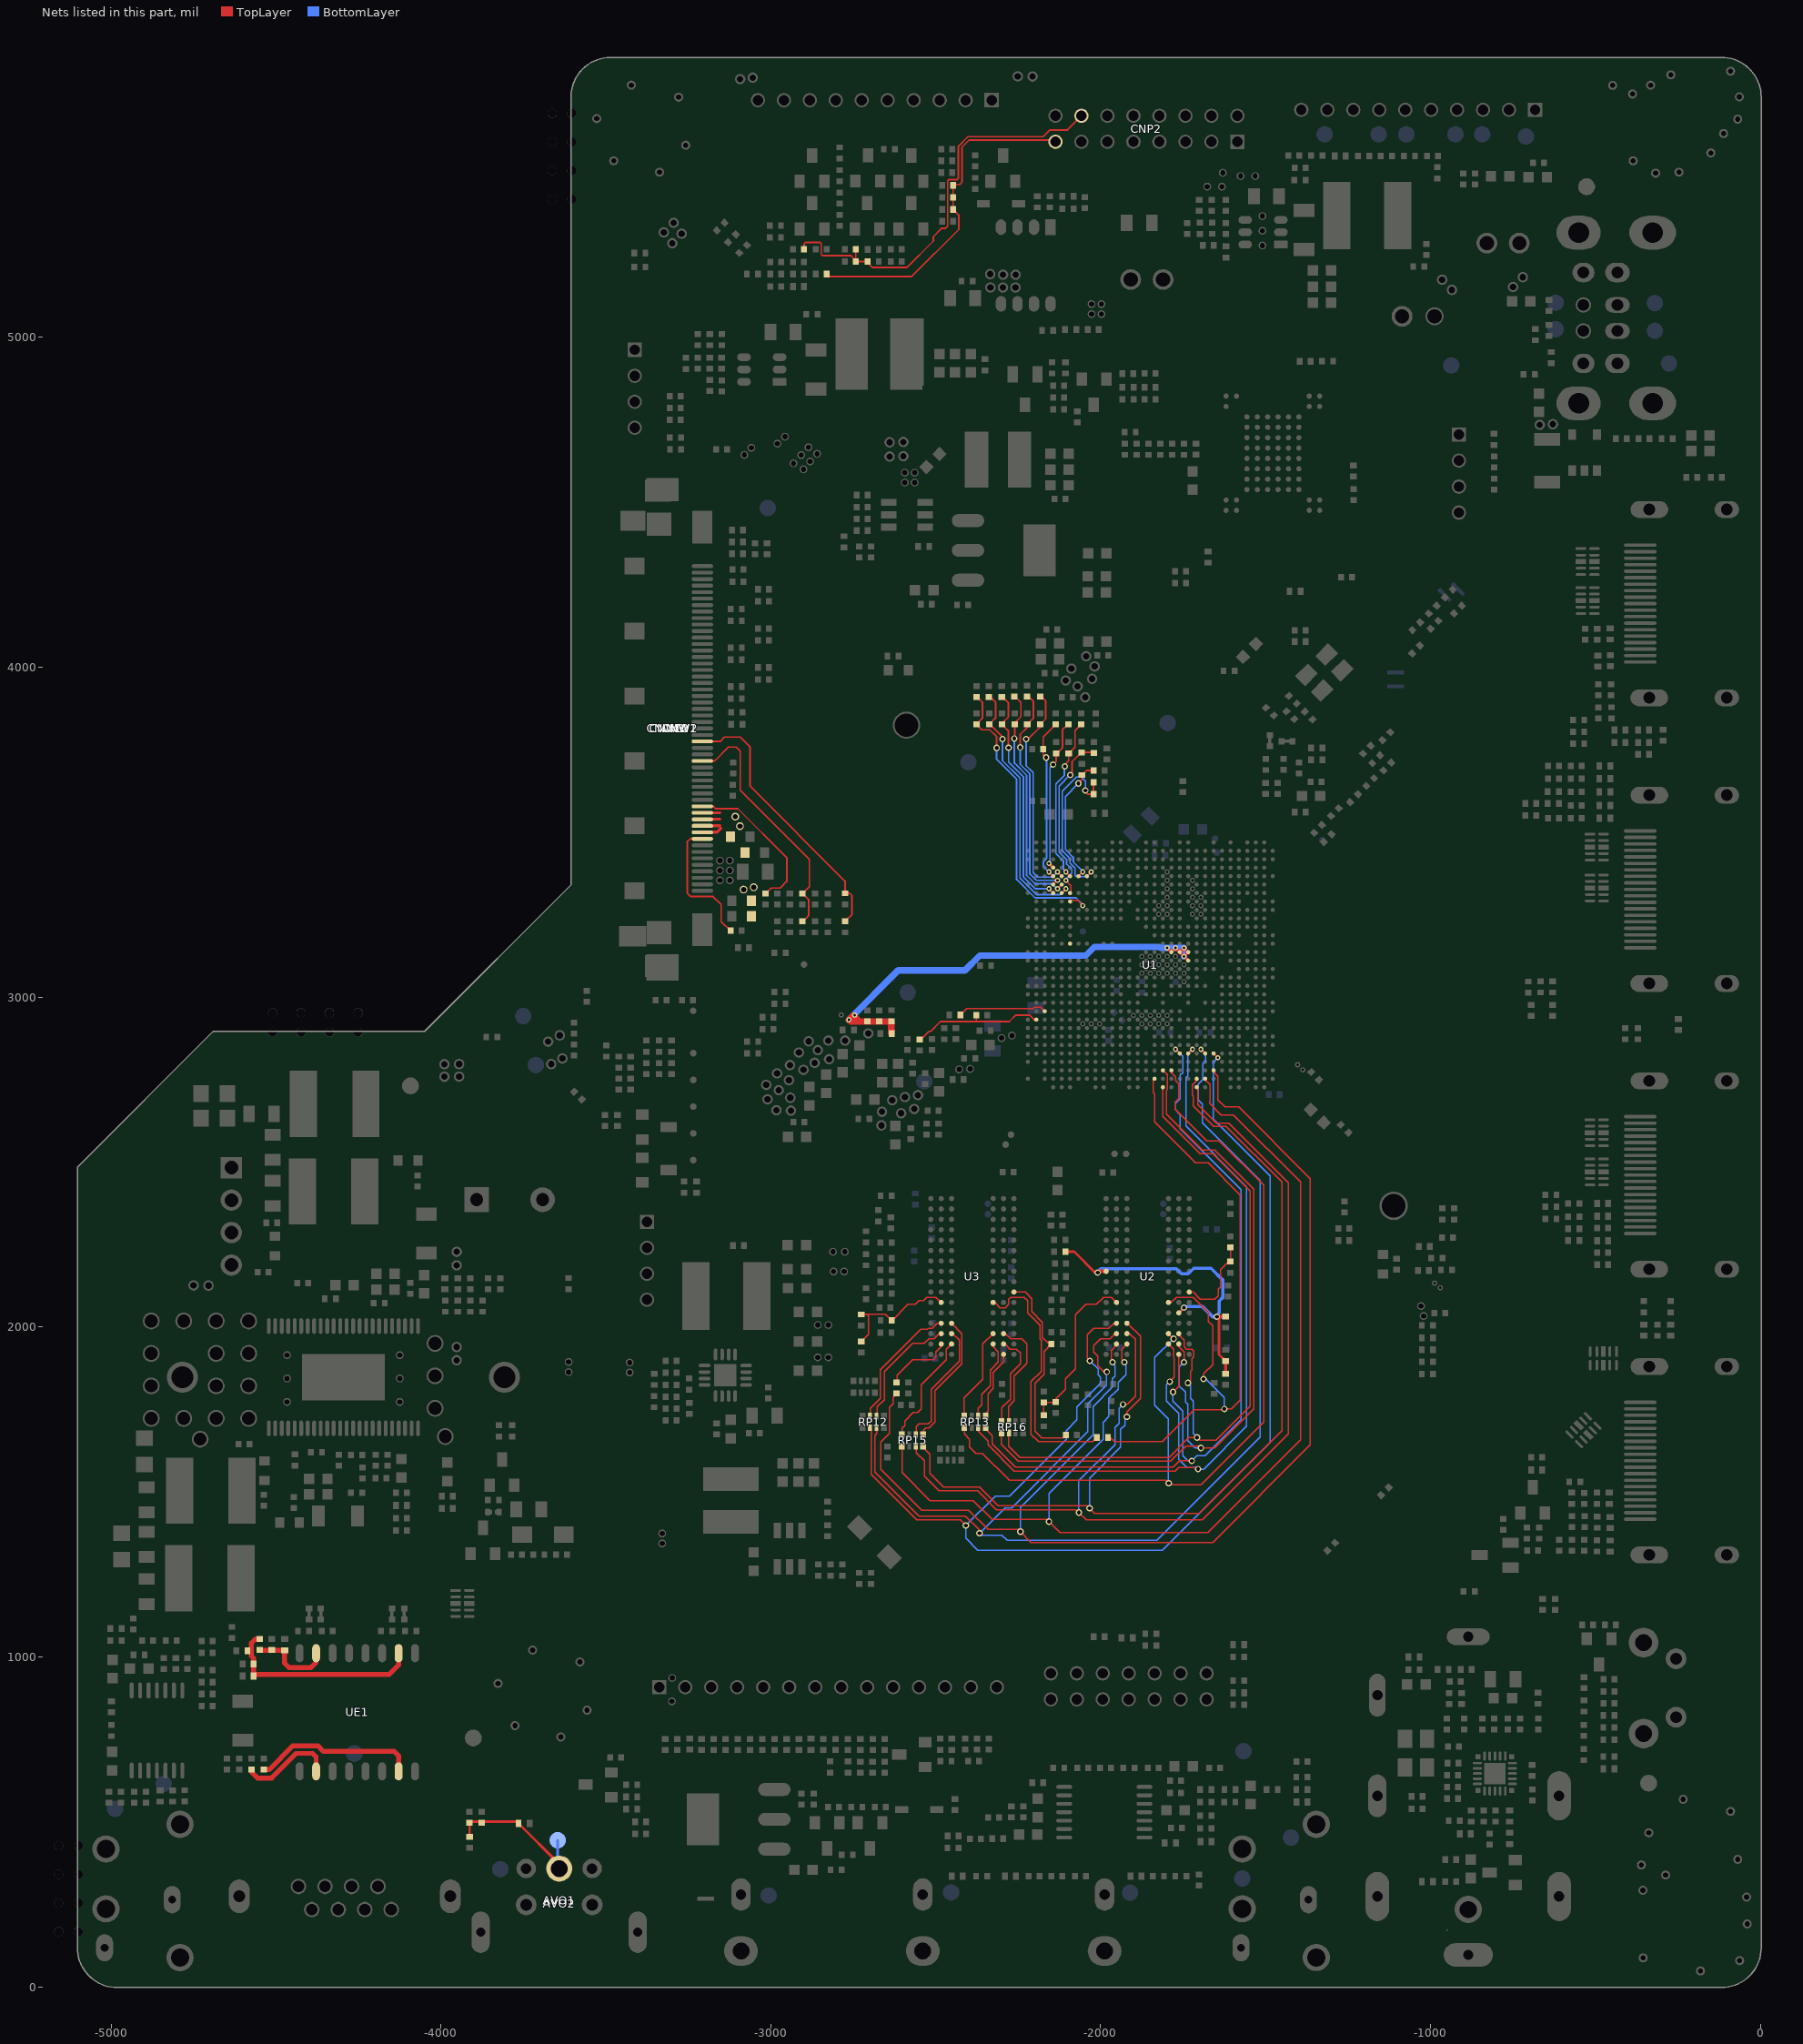
[diagram p0: the nets of this part, all layers, seen from the top]
# Altium PCB MISC86290.PcbDoc (part 11 of 31)
Units mil, origin at the board's own origin, x right, y up, seen from the top; angles counter-clockwise.
Board outline 5104.71 x 5851.49 mil, 2 copper layers (TopLayer, BottomLayer), stack 61.855 mil thick; 1026 components, 667 nets, 4280 pads, 2294 vias.

## Via types
v1: diameter 19.68, hole 11.81, TopLayer to BottomLayer, tented both sides, 1189 vias
v2: diameter 19.68/19.68 (per signal layer), hole 11.81, TopLayer to BottomLayer, tented both sides, 366 vias
v3: diameter 15.75, hole 7.87, TopLayer to BottomLayer, tented both sides, 348 vias
v4: diameter 23.62, hole 15.75, TopLayer to BottomLayer, tented both sides, 309 vias
v5: diameter 15.75/15.75 (per signal layer), hole 7.87, TopLayer to BottomLayer, tented both sides, 59 vias
v6: diameter 24/24 (per signal layer), hole 16, TopLayer to BottomLayer, tented both sides, 23 vias

## Nets (pads, with @x,y where several pads share a name; then routed paths per layer and width w, separated by ;. In a path a pad name is that pad's centre, name@x,y a point inside that pad or via, vN(x,y) a via of type N, cw(c..) or ccw(c..) an arc to the next point about the centre after c; other vN are vias at no path point) (continued)
AVDDL_HDMI: C10.2 C11.2 C110.1 pad.VIA5@-1747.36,3123.62 pad.VIA5@-1747.36,3149.21 pad.VIA5@-1772.95,3149.21 pad.VIA5@-1798.54,3149.21 pad.VIA5@-2746.06,2945.44 pad.VIA5@-2763.06,2931.44 R1.2 U1.T11 U1.U11 U1.U12 U1.U13 | length 1485.4
  TopLayer w10: pad.VIA5@-1798.54,3149.21 U1.U13@-1785.75,3136.42 pad.VIA5@-1772.95,3149.21 U1.U12@-1760.16,3136.42 ; U1.T11@-1734.57,3110.83 pad.VIA5@-1747.36,3123.62 ; U1.U12@-1760.16,3136.42 pad.VIA5@-1747.36,3123.62 ; U1.U12@-1760.16,3136.42 pad.VIA5@-1747.36,3149.21 U1.U11@-1734.57,3136.42 pad.VIA5@-1747.36,3123.62
  TopLayer w12: R1.2@-2634,2889.5 R1.2@-2634,2890.43
  TopLayer w20: pad.VIA5@-2750.5,2944 pad.VIA5@-2763.06,2931.44 -2757.73,2926.11 -2730.5,2926.11 ; pad.VIA5@-2748.39,2944 -2730.5,2926.11 ; R1.2@-2634.93,2890.43 -2634.93,2926.11 C11.2@-2707.03,2926.11 -2730.5,2926.11
  BottomLayer w19.68: pad.VIA5@-2764,2931 -2614,3081 -2411.76,3081 -2366.72,3126.03 -2045.72,3126.03 -2019.22,3152.53 -1822.04,3152.53 ; -1818.72,3149.21 pad.VIA5@-1798.54,3149.21 pad.VIA5@-1772.95,3149.21 pad.VIA5@-1747.36,3149.21 pad.VIA5@-1747.36,3123.62
B-CKE: R45.2 U1.K28 | length 271.4
  TopLayer w3.94: -2207.22,2965.53 -2205.22,2965.53 -2200.68,2970.08 -2182.4,2970.08 U1.K28@-2169.61,2957.28
  TopLayer w5: R45.2@-2425.72,2946.03 -2406.22,2965.53 -2207.22,2965.53
B-RSTZ: C60.2 R44.1 U1.J29 | length 404.3
  TopLayer w5: R44.1@-2544.85,2871.57 -2519.92,2896.5 -2515,2896.5 -2485.47,2926.03 ; -2484.22,2926.03 -2376.91,2926.03 ; C60.2@-2376.91,2945.53 -2376.91,2926.03 ; U1.J29@-2195.2,2931.69 -2202.39,2931.69 -2216.22,2945.53 -2257.64,2945.53 -2277.14,2926.03 -2376.91,2926.03
BIT_SEL: CNW1.28 CNW2.28 CNW3.28 CNW12.28 RW407.1 RW414.2 | length 836.6
  TopLayer w5: CNW3.28@-3207.67,3775.16 -3153.66,3775.16 -3140.48,3788.34 -3092.39,3788.34 -3062.75,3758.7 -3062.75,3639.64 -2775,3351.89 RW414.2@-2775,3314.73 -2760.73,3314.73 -2754,3308 -2754,3250.73 RW407.1@-2775,3229.73
BIT_SEL_1: CNW1.31 CNW2.31 CNW3.31 CNW12.31 RW410.1 RW417.2 | length 767.2
  TopLayer w5: CNW3.31@-3207.67,3716.1 -3170.29,3716.1 -3128.05,3758.34 -3104.82,3758.34 -3092.75,3746.27 -3092.75,3627.21 -2883,3417.46 -2883,3335.34 RW417.2@-2904.34,3314 -2885,3294.66 -2885,3247.61 -2903.61,3229 RW410.1@-2904.34,3228.27
BL_ADIM: CG30.2 CNP2.14 RG35.1 RG39.2 RG40.2 | length 1285.2
  TopLayer w5: RG35.1@-2899.27,5267 -2899.27,5283.73 -2895,5288 -2851,5288 -2847.02,5284.02 -2847.02,5252.02 -2843,5248 -2757.32,5248 CG30.2@-2742.27,5232.95 ; RG40.2@-2742.27,5267 CG30.2@-2742.27,5232.95 ; CG30.2@-2739.32,5230 CG30.2@-2742.27,5232.95 ; CNP2.14@-2058.21,5671.74 -2100.95,5629 -2153.5,5629 -2174,5608.5 -2402.5,5608.5 -2431.25,5579.75 -2431.25,5482.75 -2435.5,5478.5 -2460.5,5478.5 -2464,5475 -2464,5337.5 -2470.5,5331 -2481.5,5331 -2507.34,5305.16 -2507.34,5292.16 -2587.5,5212 -2691.18,5212 -2709.18,5230 CG30.2@-2742.27,5230 CG30.2@-2742.27,5232.95
BL_ON: CG1.2 CNP2.15 RG3.1 RG4.2 RG5.1 | length 1039.4
  TopLayer w5: RG5.1@-2830.27,5192 -2823.27,5185 -2572.74,5185 -2429.84,5327.9 -2429.84,5370.17 RG3.1@-2447.52,5387.84 -2447.52,5462.73 CG1.2@-2449.52,5460.73 ; CG1.2@-2447.52,5463.84 -2427.16,5463.84 -2420.43,5470.57 -2420.43,5576.43 -2398.36,5598.5 -2157.12,5598.5 -2155.62,5600 -2143.95,5600 CNP2.15@-2136.95,5593
BOARD_ID0: R19.1 R27.2 U1.AF24 | length 398.2
  TopLayer w3.94: U1.AF24@-2067.24,3366.73 v3(-2054.45,3379.53)
  TopLayer w5: v1(-2067.56,3647.77) -2057,3658.33 R27.2@-2057,3673.27 -2043.27,3687 R19.1@-2021.73,3687
  BottomLayer w5: v1@-2068,3644.39 v1@-2068,3647.33 ; v1(-2067.56,3647.77) v1@-2068,3647.33 ; v3(-2054.45,3379.53) -2054.45,3381.34 -2083.11,3410 -2083.11,3423.52 -2106.95,3447.36 -2106.95,3608.38 v1@-2068,3647.33
BOARD_ID1: R18.1 R26.2 U1.AD26 | length 786.6
  TopLayer w3.94: U1.AD26@-2118.43,3315.55 v3(-2105.63,3328.35)
  TopLayer w5: R18.1@-2330.12,3905.46 -2318.75,3894.09 -2318.75,3845.83 R26.2@-2337.75,3826.83 -2335.83,3826.83 -2294.56,3785.56 v1(-2298,3782.11) v1@-2298,3783.78
  BottomLayer w3.94: -2119.41,3314.57 v3(-2105.63,3328.35)
  BottomLayer w5: v1(-2298,3782.11) -2298,3717.54 -2244.72,3664.26 -2244.72,3360.59 -2195.08,3310.94 -2123.03,3310.94 -2119.41,3314.57
BOARD_ID2: R17.1 R25.2 U1.AD25 | length 515.8
  TopLayer w3.94: v3(-2105.63,3353.94) -2089.88,3338.19 -2089.88,3318.5 U1.AD25@-2092.83,3315.55
  TopLayer w5: v1(-2092.5,3673.5) -2087,3679 -2087,3713.27 R25.2@-2058.5,3741.77 ; R25.2@-2058,3742.27 R17.1@-2023.46,3742.27
  BottomLayer w5: v3@-2105.63,3357.79 -2087.65,3375.76 -2087.65,3387.76 -2103,3403.11 -2103,3416.63 -2125.89,3439.52 -2125.89,3640.11 v1(-2092.5,3673.5)
BOARD_ID3: R16.1 R24.2 U1.AF25 | length 508.8
  TopLayer w3.94: v3(-2105.63,3379.53) U1.AF25@-2092.83,3366.73
  TopLayer w5: v1@-2111.5,3702 -2097,3716.5 R24.2@-2097,3739.27 -2078,3758.27 -2078,3808.27 R16.1@-2059,3827.27
  BottomLayer w5: v1(-2109,3699.5) -2109.84,3698.66 -2109.84,3672.66 -2135.89,3646.61 -2135.89,3435.38 -2113,3412.49 -2113,3386.9 v3(-2105.63,3379.53)
BOARD_ID4: R15.1 R23.2 U1.AD27 | length 693.8
  TopLayer w3.94: v3(-2156.81,3328.35) U1.AD27@-2144.02,3315.55
  TopLayer w5: R23.2@-2298.75,3826.83 -2280.14,3808.23 -2280.14,3757.25 v1(-2279,3756.11) ; R23.2@-2298.75,3830.83 -2279.75,3849.83 -2279.75,3891.86 -2294.72,3906.83 R15.1@-2298.75,3906.83
  BottomLayer w5: v1(-2279,3756.11) -2279,3712.68 -2234.72,3668.4 -2234.72,3364.78 -2198.29,3328.35 v3(-2156.81,3328.35)
BOARD_ID5: R14.1 R22.2 U1.AE27 | length 676
  TopLayer w3.94: U1.AE27@-2144.02,3341.14 v3(-2131.22,3353.94)
  TopLayer w5: v1(-2244,3757.11) -2244,3796.58 -2222.75,3817.83 ; R22.2@-2222.75,3826.83 -2203.75,3845.83 -2203.75,3896.47 -2214.11,3906.83 R14.1@-2222.75,3906.83
  BottomLayer w5: v1(-2244,3757.11) -2244,3705.96 -2214.72,3676.69 -2214.72,3373.16 -2195.5,3353.94 v3(-2131.22,3353.94)
BOARD_ID6: R13.1 R21.2 U1.AC25 | length 912.6
  TopLayer w3.94: U1.AC25@-2092.83,3289.96 -2089.88,3292.91 -2070.2,3292.91 v3(-2054.45,3277.17)
  TopLayer w5: R13.1@-2370.55,3905.95 -2358.63,3894.03 -2358.63,3844.95 R21.2@-2376.75,3826.83 -2360.39,3810.47 -2336.47,3810.47 -2315.34,3789.34 v1(-2315.34,3755.45) v1@-2318.55,3758.66
  BottomLayer w5: v1(-2315.34,3755.45) -2315.34,3720.74 -2254.72,3660.12 -2254.72,3356.4 -2199.27,3300.94 -2074.38,3300.94 -2054.45,3281.01 v3(-2054.45,3277.17)
BOARD_ID7: R12.1 R20.2 U1.AE26 | length 685.7
  TopLayer w3.94: v3(-2131.22,3328.35) U1.AE26@-2118.43,3341.14
  TopLayer w5: v1@-2260.75,3785.36 -2260.75,3817.83 ; R20.2@-2260.75,3830.83 -2241.75,3849.83 -2241.75,3893.46 -2255.12,3906.83 R12.1@-2260.75,3906.83
  BottomLayer w5: v1@-2261.66,3783.45 -2261.66,3709.48 -2224.72,3672.55 -2224.72,3368.97 -2199.49,3343.74 -2146.61,3343.74 v3(-2131.22,3328.35)
  other v1: -2262,3784.11
BOOT_CTL: U1.V25
CNW12_PIN38: CNW1.38 CNW2.38 CNW3.38 CNW12.38 RW389.2 | length 472.7
  TopLayer w5: CNW3.38@-3207.67,3578.31 -3174.5,3578.31 -3167.57,3571.37 -3100.37,3571.37 -2951.5,3422.5 -2951.5,3350.96 -2971.83,3330.62 -2999.5,3330.62 -3016.08,3314.04 RW389.2@-3016.5,3313.62
CNW12_PIN42: CNW1.39 CNW1.40 CNW1.41 CNW1.42 CNW2.39 CNW2.40 CNW2.41 CNW2.42 CNW3.39 CNW3.40 CNW3.41 CNW3.42 CNW12.39 CNW12.40 CNW12.41 CNW12.42 pad.VIA5@-3052,3333 pad.VIA5@-3082.5,3326 pad.VIA5@-3093.5,3518.5 pad.VIA5@-3107.5,3547.5 RW52.2 RW53.2 RW55.2 RW56.2 | length 192.8
  TopLayer w9: CNW3.42@-3201.25,3500 -3163.25,3500 -3152.25,3511 ; CNW3.41@-3201.25,3519.68 -3154.84,3519.68 ; CNW3.40@-3201.25,3539.37 -3154.84,3539.37 ; CNW3.39@-3201.25,3559.05 -3154.84,3559.05
CNW12_PIN43: CNW1.43 CNW2.43 CNW3.43 CNW12.43 RW26.1 | length 416.6
  TopLayer w5: CNW3.43@-3205.47,3477.69 CNW3.43@-3207.67,3479.88 -3244.62,3479.88 -3253.5,3471 -3253.5,3315.5 -3243,3305 -3175,3305 -3150.5,3280.5 -3150.5,3229 -3123.5,3202 RW26.1@-3122.23,3202
COAX: AVO1.1 AVO2.2 CO1.2 CO2.2 COAX.1 DO1.K RO3.2 | length 467
  TopLayer w8: CO1.2@-3913.25,454.73 -3913.25,494.58 -3907.56,500.27 -3770.25,500.27 DO1.K@-3764.98,495 -3642.98,373 AVO1.1@-3642.98,358.27
  BottomLayer w8: COAX.1@-3646.25,444 -3646.25,361.53 AVO1.1@-3642.98,358.27
CRD: CE6.1 DE2.K RE6.2 UE1.7 | length 252.5
  TopLayer w15: RE6.2@-4549.6,1021.2 -4548.64,1020.24 DE2.K@-4474.46,1020.24 ; DE2.K@-4474.46,1021.23 DE2.K@-4474.46,1020.24 ; DE2.K@-4473.96,1020.24 DE2.K@-4474.46,1020.24 ; UE1.7@-4378.5,1011.13 -4378.5,983.22 -4394.72,967 -4460.28,967 -4474.46,981.18 DE2.K@-4474.46,1020.24
CRX: RE1.2 UE1.10 | length 290.2
  TopLayer w15: RE1.2@-4574.17,658.5 -4574.17,650.67 -4556,632.5 -4513.5,632.5 -4438.66,707.34 -4389.34,707.34 -4378.5,696.5 UE1.10@-4378.5,652.87
CTD: CE7.2 CE8.2 DE1.K RE6.1 UE1.2 | length 621.7
  TopLayer w15: DE1.K@-4567.96,947 DE1.K@-4567.86,947 ; DE1.K@-4567.46,941 DE1.K@-4567.86,941.4 DE1.K@-4567.86,947 ; RE6.1@-4549.6,1054.67 -4561.68,1054.67 -4575,1041.35 -4575,1003 -4567.53,995.53 -4567.53,980.4 -4567.86,980.07 DE1.K@-4567.86,947 ; UE1.2@-4128.5,1011.13 -4128.5,975.22 -4156.72,947 DE1.K@-4567.86,947
CTX: RE2.2 UE1.15 | length 497.8
  TopLayer w15: RE2.2@-4536.67,658.31 -4521.19,658.31 -4449,730.5 -4373.5,730.5 -4356,713 -4141.5,713 -4128.5,700 UE1.15@-4128.5,652.87
CUST_ID0: R7.1 R11.2 U1.AF23 | length 536
  TopLayer w3.94: U1.AF23@-2041.65,3366.73 v3(-2028.86,3379.53)
  TopLayer w5: v1(-2046.43,3626.64) -2046.43,3622.43 -2039,3615 R11.2@-2021.73,3615 R7.1@-2021.73,3651
  BottomLayer w3.94: v1@-2046.43,3626.57 v1(-2046.43,3626.64) -2046.43,3654.94 -2059,3667.5 -2073.5,3667.5 -2116.42,3624.58 -2116.42,3443.44 -2093.53,3420.55 -2093.53,3407.03 -2078.18,3391.68 -2078.18,3369.14 -2073.72,3364.68 -2043.7,3364.68 v3(-2028.86,3379.53)
CUST_ID1: R6.1 R10.2 U1.AF26 | length 673.8
  TopLayer w3.94: v3(-2131.22,3379.53) U1.AF26@-2118.43,3366.73
  TopLayer w5: v1(-2226,3782) -2225,3781 -2220.81,3781 -2183.75,3818.06 ; R10.2@-2183.75,3827.06 -2166.4,3844.4 -2166.4,3897.31 -2176.15,3907.06 R6.1@-2183.75,3907.06
  BottomLayer w5: v1(-2226,3782) -2226,3702.1 -2204.72,3680.83 -2204.72,3377.35 -2191.4,3364.03 -2146.72,3364.03 v3(-2131.22,3379.53)
CUST_ID2: R5.1 R9.2 U1.AG27 | length 465.3
  TopLayer w5: v1@-2144.31,3702.31 v1(-2144.31,3705.06) -2135,3714.37 R9.2@-2135,3739.27 -2132.05,3739.27 -2116,3755.32 -2116,3810.25 -2098.98,3827.27 R5.1@-2098,3827.27
  TopLayer w10: v3(-2156.81,3405.12) U1.AG27@-2144.02,3392.32
  BottomLayer w5: v3@-2153.72,3408.2 -2153.72,3695.65 v1(-2144.31,3705.06)
CUST_ID3: R4.1 R8.2 U1.AF27 | length 491.5
  TopLayer w3.94: v3(-2156.81,3379.53) U1.AF27@-2144.02,3366.73
  TopLayer w5: R8.2@-2174.27,3752 -2174.27,3735.02 v1(-2165.56,3726.32) ; R8.2@-2174.27,3758 -2174.27,3789 R4.1@-2136,3827.27
  BottomLayer w5: v1(-2165.56,3726.32) -2165.88,3726 -2163.72,3723.85 -2163.72,3422.03 -2173.72,3412.03 -2173.72,3396.44 v3(-2156.81,3379.53)
D-CSB1: R53.1 R65.2 R118.1 U2.L2 | length 517.7
  TopLayer w3.94: R65.2@-2172.56,1732.2 R118.1@-2172.56,1770.94 -2137.76,1770.94 R53.1@-2136.3,1772.4 -2136.3,1781.93 -2106.61,1811.61 -2106.61,1843.11 -2076.1,1873.62 -2076.1,2037.01 -2044.61,2068.5 -2013.11,2068.5 -1991.46,2090.16 -1967.83,2090.16 U2.L2@-1952.09,2074.41
D-CSB2: R57.2 R101.1 R102.2 U3.L2 | length 376.5
  TopLayer w3.94: R102.2@-2724.72,2038.03 -2716.18,2038.98 -2709.72,2038.98 ; R57.2@-2723.74,1958.35 -2704.06,1978.03 -2704.06,2033.31 -2709.72,2038.98 ; U3.L2@-2483.58,2074.41 -2499.33,2090.16 -2526.89,2090.16 -2536.73,2080.31 -2550.51,2080.31 -2562.32,2068.5 -2583.98,2068.5 -2632.65,2019.83 -2632.83,2019.39 -2632.87,2019.29 -2652.56,2038.98 -2709.72,2038.98
D-DDR3-CKE-T1: R52.1 R62.2 U2.K9 | length 263.5
  TopLayer w3.94: U2.K9@-1731.61,2105.91 -1719.8,2105.91 -1698.15,2084.25 -1653.86,2084.25 -1644.02,2094.09 -1644.02,2114.76 -1637.13,2121.65 -1637.13,2174.13 -1606.61,2204.65 R62.2@-1606.61,2241.42
D-DDR3-CKE-T2: R56.2 R108.2 U3.K9 | length 619.1
  TopLayer w3.94: U3.K9@-2263.11,2105.91 -2228.66,2105.91 -2208.98,2086.22 -2208.98,2046.85 -2176.5,2014.37 -2176.5,1968.11 -2156.81,1948.43 R108.2@-2149.25,1948.43 -2171.57,1926.1 -2171.57,1856.89 -2199.13,1829.33 -2199.13,1684.65 -2178.46,1663.98 -2114.8,1663.98 R56.2@-2105.94,1672.83
D-MVREFCA-T1: C98.2 C99.2 R66.1 R67.2 U2.H1 U2.M8 | length 1027.4
  TopLayer w7.87: C98.2@-2105.32,2227.95 -2080.04,2227.95 -2017.05,2164.96 v2(-2009.17,2164.96) ; U2.M8@-1763.11,2042.91 v2(-1747.36,2058.66) ; v2(-1647.95,2031.1) -1641.06,2024.21 -1641.06,1916.61 R67.2@-1621.38,1896.93
  TopLayer w9.84: v2(-2009.17,2164.96) -2007.2,2164.96 -2003.27,2168.9 U2.H1@-1983.58,2168.9 ; v2(-1647.95,2031.1) -1621.69,2031.1 C99.2@-1621.38,2031.42 ; R66.1@-1621.38,1858.19 R67.2@-1621.38,1896.93
  BottomLayer w9.84: v2(-2009.17,2164.96) -2001.3,2174.8 -1999.33,2176.77 -1770.98,2176.77 -1755.24,2161.02 -1734.57,2161.02 -1717.83,2177.76 -1665.67,2177.76 -1629.25,2141.34 -1629.25,2090.16 -1641.06,2078.35 -1641.06,2042.91 v2(-1647.95,2031.1) -1660.75,2031.1 -1692.24,2062.6 -1743.43,2062.6 v2(-1747.36,2058.66)
D_DDR3_A0: RP15.2 U1.B10 U2.N3 | length 3160.4
  TopLayer w3.94: RP15.2@-2536.73,1638.39 -2536.73,1633.46 -2517.05,1613.78 -2517.05,1555.71 -2476.69,1515.35 -2367.44,1515.35 -2310.35,1458.27 -2041.65,1458.27 v2(-2033.78,1450.39) -2018.03,1434.65 -1702.09,1434.65 -1451.1,1685.63 -1451.1,2439.57 -1619.41,2607.87 -1656.81,2607.87 -1719.8,2670.87 -1719.8,2700.39 -1721.77,2702.36 -1721.77,2733.86 -1709.96,2745.67 -1709.96,2751.57 U1.B10@-1708.98,2752.56 ; v2(-1920.59,1727.95) -1920.59,1741.73 -1879.25,1783.07 -1879.25,1972.05 -1918.62,2011.42 U2.N3@-1920.59,2011.42
  BottomLayer w3.94: v2(-2033.78,1450.39) -2033.78,1540.94 -1939.29,1635.43 -1939.29,1689.57 -1926.5,1702.36 -1926.5,1722.05 v2(-1920.59,1727.95)
D_DDR3_A0_H: RP15.1 U3.N3 | length 396.6
  TopLayer w3.94: RP15.1@-2536.73,1681.69 -2536.73,1686.61 -2529.84,1693.5 -2520,1693.5 -2502.28,1711.22 -2502.28,1806.69 -2420.59,1888.39 -2420.59,1979.92 U3.N3@-2452.09,2011.42
D_DDR3_A1: RP13.8 U1.C13 U2.P7 | length 2799.3
  TopLayer w3.94: RP13.8@-2413.7,1694.49 -2413.53,1688.55 -2413.53,1675.62 -2397.95,1660.04 -2397.95,1636.42 -2378.27,1616.73 -2358.58,1616.73 -2276.89,1535.04 -1802.48,1535.04 v2(-1793.62,1526.18) -1788.7,1521.26 -1696.18,1521.26 -1506.22,1711.22 -1506.22,2429.72 -1641.06,2564.57 -1678.46,2564.57 -1774.92,2661.02 -1774.92,2680.71 -1763.11,2692.52 -1763.11,2737.8 -1772.95,2747.64 -1772.95,2758.51 -1785.22,2770.77 -1785.75,2771.26 U1.C13@-1785.75,2778.15 ; U2.P7@-1794.61,1979.92 v2(-1778.86,1964.17)
  BottomLayer w3.94: v2(-1793.62,1526.18) -1795.59,1528.15 -1795.59,1648.23 -1794.61,1649.21 -1794.61,1722.05 -1835.94,1763.39 -1835.94,1907.09 v2(-1778.86,1964.17)
D_DDR3_A1_H: RP13.7 U3.P7 | length 278.4
  TopLayer w3.94: RP13.7@-2413.7,1737.8 -2413.7,1785.04 -2357.6,1841.14 -2357.6,1948.43 U3.P7@-2326.1,1979.92
D_DDR3_A2: RP15.4 U1.A10 U2.P3 | length 3192.3
  TopLayer w3.94: RP15.4@-2559.37,1638.39 -2559.37,1618.7 -2534.76,1594.09 -2534.76,1547.83 -2490.47,1503.54 -2373.35,1503.54 -2316.26,1446.46 -2075.12,1446.46 v2(-2066.26,1437.6) -2043.62,1414.96 -1692.24,1414.96 -1431.42,1675.79 -1431.42,2437.6 -1611.54,2617.72 -1648.94,2617.72 -1705.04,2673.82 -1705.04,2723.03 U1.A10@-1708.98,2726.97 ; v2(-1932.4,1765.35) -1933.39,1765.35 -1932.5,1765.65 -1930.43,1766.34 -1919.61,1766.34 -1895,1790.94 -1895,1962.2 -1912.72,1979.92 U2.P3@-1920.59,1979.92
  BottomLayer w3.94: v2(-2066.26,1437.6) -2066.26,1534.06 -1957.01,1643.31 -1957.01,1695.47 -1944.21,1708.27 -1944.21,1753.54 v2(-1932.4,1765.35)
D_DDR3_A2_H: RP15.3 U3.P3 | length 380.7
  TopLayer w3.94: RP15.3@-2559.37,1681.69 -2559.37,1697.44 -2550.51,1706.3 -2522.95,1706.3 -2514.09,1715.16 -2514.09,1811.61 -2428.46,1897.24 -2428.46,1960.24 -2448.15,1979.92 U3.P3@-2452.09,1979.92
D_DDR3_A3: RP12.6 U1.E8 U2.N2 | length 3758.8
  TopLayer w3.94: RP12.6@-2698.15,1694.49 -2696.18,1692.52 -2696.18,1552.76 -2558.39,1414.96 -2425.51,1414.96 v2(-2408.78,1398.23) ; v2(-2032.8,1897.24) -2040.67,1905.12 -2040.67,1975.98 -2020.98,1995.67 -1975.71,1995.67 -1959.96,2011.42 U2.N2@-1952.09,2011.42 ; U1.E8@-1657.8,2829.33 v5(-1645,2816.54)
  BottomLayer w3.94: v2(-2032.8,1897.24) -2008.19,1872.64 -2008.19,1854.92 -2000.32,1847.05 -2000.32,1829.33 -2072.17,1757.48 -2072.17,1718.11 -2104.65,1685.63 -2104.65,1659.06 -2275.91,1487.8 -2319.21,1487.8 v2(-2408.78,1398.23) -2408.78,1359.84 -2372.36,1323.43 -1813.31,1323.43 -1486.54,1650.2 -1486.54,2458.27 -1658.78,2630.51 -1658.78,2802.76 v5(-1645,2816.54)
D_DDR3_A3_H: RP12.5 U3.N2 | length 387.9
  TopLayer w3.94: RP12.5@-2698.15,1737.8 -2698.15,1753.54 -2667.64,1784.06 -2667.64,1870.67 -2544.61,1993.7 -2524.92,1993.7 -2522.95,1995.67 -2511.14,1995.67 -2495.39,2011.42 U3.N2@-2483.58,2011.42
D_DDR3_A4: RP16.6 U1.A14 U2.P8 | length 2315.3
  TopLayer w3.94: RP16.6@-2278.86,1678.74 -2278.86,1639.37 -2244.41,1604.92 -1792.64,1604.92 -1732.6,1664.96 v2(-1707.99,1664.96) -1700.12,1657.09 -1650.91,1657.09 -1547.56,1760.43 -1547.56,2412.01 -1660.75,2525.2 -1698.15,2525.2 -1811.34,2638.39 U1.A14@-1811.34,2726.97 ; U2.P8@-1763.11,1979.92 -1763.11,1975.98 -1747.36,1960.24 -1747.36,1940.55 -1739.49,1932.68 -1723.74,1932.68 -1717.83,1926.77 -1717.83,1910.04 -1723.74,1904.13 -1723.74,1869.69 -1727.68,1865.75 -1727.68,1838.19 v2(-1735.55,1830.31)
  BottomLayer w3.94: v2(-1735.55,1830.31) -1727.68,1822.44 -1727.68,1783.07 -1719.8,1775.2 -1719.8,1676.77 v2(-1707.99,1664.96)
D_DDR3_A4_H: RP16.5 U3.P8 | length 333.1
  TopLayer w3.94: U3.P8@-2294.61,1979.92 -2288.7,1979.92 -2272.95,1964.17 -2239.49,1964.17 -2223.74,1948.43 -2223.74,1889.37 -2262.13,1850.98 -2262.13,1776.18 -2278.86,1759.45 RP16.5@-2278.86,1722.05
D_DDR3_A5: RP12.4 U1.E9 U2.P2 | length 3660
  TopLayer w3.94: RP12.4@-2678.46,1694.49 -2678.46,1676.77 -2684.37,1670.87 -2684.37,1560.63 -2550.51,1426.77 -2409.76,1426.77 -2367.44,1384.45 v2(-2367.44,1374.61) ; v2(-1981.61,1863.78) -1989.49,1863.78 -2009.17,1883.46 -2009.17,1912.01 -2021.97,1924.8 -2021.97,1943.5 -2001.3,1964.17 -1971.77,1964.17 -1956.02,1979.92 U2.P2@-1952.09,1979.92 ; v5(-1696.18,2842.13) U1.E9@-1683.39,2829.33
  BottomLayer w3.94: v2(-1981.61,1863.78) -1982.6,1862.8 -1982.6,1823.43 -2038.7,1767.32 -2038.7,1682.68 -2270,1451.38 -2290.67,1451.38 v2(-2367.44,1374.61) -2361.54,1368.7 -2299.53,1368.7 -2283.78,1352.95 -1829.06,1352.95 -1516.06,1665.94 -1516.06,2444.49 -1691.26,2619.68 -1691.26,2675.79 -1704.06,2688.58 -1704.06,2735.83 -1690.28,2749.61 -1690.28,2797.83 -1682.4,2805.71 -1682.4,2828.35 v5(-1696.18,2842.13)
D_DDR3_A5_H: RP12.3 U3.P2 | length 356.3
  TopLayer w3.94: RP12.3@-2678.46,1737.8 -2677.53,1738.73 -2677.53,1758.42 -2655.83,1780.12 -2655.83,1864.76 -2570.41,1950.18 -2534.98,1950.18 -2520.98,1964.17 -2505.24,1964.17 -2489.49,1979.92 U3.P2@-2483.58,1979.92
D_DDR3_A6: RP16.8 U1.C14 U2.R8 | length 2420.9
  TopLayer w3.94: RP16.8@-2301.5,1678.74 -2301.5,1644.29 -2250.32,1593.11 -1787.72,1593.11 -1741.46,1639.37 -1702.09,1639.37 v2(-1696.18,1633.46) -1654.84,1633.46 -1535.75,1752.56 -1535.75,2417.91 -1654.84,2537.01 -1692.24,2537.01 -1800.51,2645.28 -1800.51,2718.11 -1798.54,2720.08 -1798.54,2765.35 U1.C14@-1811.34,2778.15 ; U2.R8@-1763.11,1948.43 -1763.11,1940.55 -1747.36,1924.8 v2(-1747.36,1893.31)
  BottomLayer w3.94: v2(-1747.36,1893.31) -1762.13,1878.54 -1762.13,1821.46 -1743.43,1802.76 -1743.43,1773.23 -1735.55,1765.35 -1735.55,1655.12 -1713.9,1633.46 v2(-1696.18,1633.46)
D_DDR3_A6_H: RP16.7 U3.R8 | length 285.5
  TopLayer w3.94: RP16.7@-2301.5,1722.05 -2299.7,1723.85 -2299.7,1755.34 -2273.94,1781.1 -2273.94,1857.87 -2243.43,1888.39 -2243.43,1920.87 -2255.24,1932.68 -2274.92,1932.68 -2290.67,1948.43 U3.R8@-2294.61,1948.43
D_DDR3_A7: R58.1 U1.C8 U2.R2 | length 3751.4
  TopLayer w3.94: R58.1@-2617.44,1798.5 -2629.25,1786.69 -2629.25,1767.32 -2640.08,1756.5 -2640.08,1677.76 -2666.65,1651.18 -2666.65,1568.5 -2542.64,1444.49 -2399.92,1444.49 -2341.85,1386.42 -2250.32,1386.42 v2(-2243.43,1379.53) -2210.94,1347.05 -1659.76,1347.05 -1364.49,1642.32 -1364.49,2449.41 -1582.01,2666.93 -1623.35,2666.93 -1645,2688.58 -1645,2760.47 U1.C8@-1657.75,2773.23 ; v2(-1963.9,1893.31) -1967.83,1891.34 -1967.83,1928.74 -1952.09,1944.49 U2.R2@-1952.09,1948.43 ; U1.C8@-1657.8,2773.23 U1.C8@-1657.8,2778.15
  BottomLayer w3.94: v2(-2243.43,1379.53) -2243.43,1452.36 -2022.95,1672.83 -2022.95,1759.45 -1964.88,1817.52 -1964.88,1843.11 -1957.01,1850.98 -1957.01,1882.48 -1963.9,1889.37 v2(-1963.9,1893.31)
D_DDR3_A7_H: R58.2 U3.R2 | length 202.3
  TopLayer w3.94: R58.2@-2617.44,1838.5 -2617.44,1853.94 -2570.2,1901.18 -2507.2,1901.18 -2499.33,1909.06 -2499.33,1924.8 -2483.58,1940.55 U3.R2@-2483.58,1948.43
D_DDR3_A8: RP13.2 U1.E12 U2.T8 | length 2503.2
  TopLayer w3.94: RP13.2@-2348.74,1694.49 -2348.74,1689.57 -2329.06,1669.88 -2329.06,1646.26 -2258.19,1575.39 -1779.84,1575.39 -1761.14,1594.09 v2(-1723.74,1594.09) ; v2(-1780.83,1802.76) -1764.09,1819.49 -1764.09,1915.94 U2.T8@-1763.11,1916.93 ; v5(-1772.95,2842.13) U1.E12@-1760.16,2829.33
  BottomLayer w3.94: v2(-1780.83,1802.76) -1780.83,1775.2 -1751.3,1745.67 -1751.3,1609.84 -1735.55,1594.09 v2(-1723.74,1594.09) -1707.99,1609.84 -1683.39,1609.84 -1575.12,1718.11 -1575.12,2416.93 -1759.17,2600.98 -1759.17,2644.29 -1774.92,2660.04 -1774.92,2676.77 -1759.17,2692.52 -1759.17,2763.39 -1751.3,2771.26 -1751.3,2820.47 v5(-1772.95,2842.13)
D_DDR3_A8_H: RP13.1 U3.T8 | length 201.6
  TopLayer w3.94: RP13.1@-2348.74,1737.8 -2341.85,1744.68 -2341.85,1797.83 -2326.1,1813.58 -2326.1,1861.81 -2294.61,1893.31 U3.T8@-2294.61,1916.93
D_DDR3_A9: RP15.8 U1.B9 U2.R3 | length 3363.8
  TopLayer w3.94: RP15.8@-2601.69,1638.39 -2601.69,1558.66 -2517.05,1474.02 -2386.14,1474.02 -2329.06,1416.93 -2163.7,1416.93 v2(-2156.81,1410.04) -2123.35,1376.57 -1675.51,1376.57 -1394.02,1658.07 -1394.02,2439.57 -1597.76,2643.31 -1598.53,2642.53 -1634.38,2642.53 -1635.16,2643.31 -1668.62,2676.77 -1668.62,2677.5 -1669.4,2678.28 -1669.4,2683.14 -1668.62,2683.92 -1668.62,2724 -1668.58,2734.59 -1683.39,2749.39 U1.B9@-1683.39,2752.56 ; v2(-1928.46,1893.31) -1936.34,1901.18 -1936.34,1932.68 U2.R3@-1920.59,1948.43
  BottomLayer w3.94: v2(-2156.81,1410.04) -2156.81,1495.67 -1992.44,1660.04 -1992.44,1711.08 -1975.71,1727.82 -1975.71,1783.07 -1947.17,1811.61 -1947.17,1831.3 -1923.54,1854.92 -1923.54,1888.39 v2(-1928.46,1893.31)
D_DDR3_A9_H: RP15.7 U3.R3 | length 336.2
  TopLayer w3.94: RP15.7@-2601.69,1681.69 -2601.69,1693.5 -2593.82,1701.38 -2593.82,1715.16 -2568.23,1740.75 -2555.43,1740.75 -2543.62,1752.56 -2543.62,1824.41 -2467.83,1900.2 -2467.83,1932.68 U3.R3@-2452.09,1948.43
D_DDR3_A10: R59.1 U1.B15 U2.L7 | length 2045.6
  TopLayer w3.94: R59.1@-1971.46,1664.96 -1971.14,1664.96 -1958.35,1652.17 -1813.31,1652.17 -1716.85,1748.62 -1628.27,1748.62 v2(-1625.32,1751.57) -1603.66,1751.57 -1577.09,1778.15 -1577.09,2400.2 -1674.53,2497.64 -1711.93,2497.64 -1835.94,2621.65 -1835.94,2706.3 -1840.87,2711.22 -1840.87,2748.62 U1.B15@-1836.93,2752.56 ; U2.L7@-1794.61,2074.41 -1786.73,2074.41 -1770.98,2090.16 -1719.8,2090.16 -1673.54,2043.9 -1673.54,2016.34 -1660.75,2003.54 -1660.75,1885.43 -1687.32,1858.86 -1687.32,1843.11 v2(-1688.31,1842.13)
  BottomLayer w3.94: v2(-1688.31,1842.13) -1680.43,1842.13 -1625.32,1787.01 v2(-1625.32,1751.57)
D_DDR3_A10_H: R59.2 U3.L7 | length 786.6
  TopLayer w3.94: U3.L7@-2326.1,2074.41 -2321.18,2074.41 -2305.43,2058.66 -2288.7,2058.66 -2278.86,2068.5 -2278.86,2084.25 -2272.95,2090.16 -2231.61,2090.16 -2221.77,2080.31 -2221.77,2042.91 -2184.37,2005.51 -2184.37,1964.17 -2180.43,1960.24 -2180.43,1864.76 -2210.94,1834.25 -2210.94,1674.8 -2188.31,1652.17 -2024.25,1652.17 R59.2@-2011.46,1664.96
D_DDR3_A11: RP13.4 U1.E11 U2.R7 | length 2640.1
  TopLayer w3.94: RP13.4@-2371.38,1694.49 -2371.38,1683.66 -2341.85,1654.13 -2341.85,1642.32 -2263.11,1563.58 -1773.94,1563.58 -1763.11,1574.41 -1709.96,1574.41 v2(-1705.04,1569.49) ; U2.R7@-1794.61,1948.43 -1778.86,1932.68 -1778.86,1907.09 -1776.89,1905.12 -1776.89,1848.03 v2(-1790.67,1834.25) ; U1.E11@-1734.57,2829.33 v5(-1721.77,2842.13)
  BottomLayer w3.94: v2(-1790.67,1834.25) -1800.51,1824.41 -1800.51,1775.2 -1763.11,1737.8 -1763.11,1599.02 -1738.5,1574.41 -1709.96,1574.41 v2(-1705.04,1569.49) -1704.06,1568.5 -1688.31,1568.5 -1557.4,1699.41 -1557.4,2424.8 -1741.46,2608.86 -1741.46,2755.51 -1735.55,2761.42 -1735.55,2828.35 v5(-1721.77,2842.13)
D_DDR3_A11_H: RP13.3 U3.R7 | length 242.4
  TopLayer w3.94: RP13.3@-2371.38,1737.8 -2371.38,1753.54 -2360.55,1764.37 -2360.55,1795.87 -2333.98,1822.44 -2333.98,1869.69 -2310.35,1893.31 -2310.35,1924.8 -2326.1,1940.55 U3.R7@-2326.1,1948.43